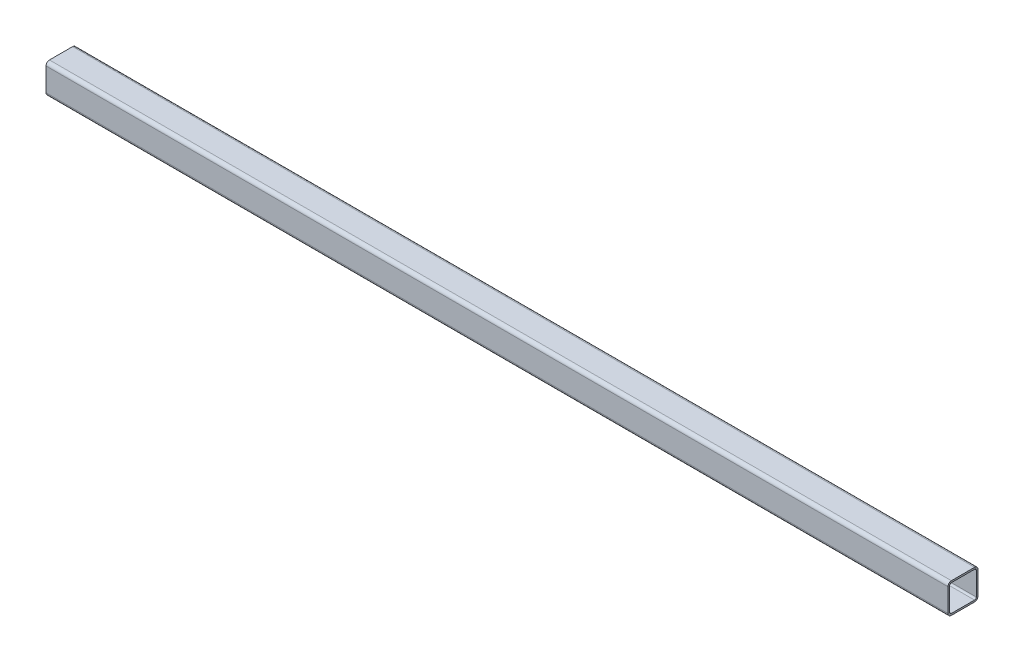
SolidWorks part; units mm, degrees
material "Q235"
ref_plane "Front" through (0, 0, 0) normal (0, 0, 1) x (1, 0, 0)
ref_plane "Top" through (0, 0, 0) normal (0, 1, 0) x (1, 0, 0)
ref_plane "Right" through (0, 0, 0) normal (1, 0, 0) x (0, 0, -1)
sketch "Sketch1" plane through (0, 0, 0) normal (0, 0, 1) x (1, 0, 0)
  line L0 (0, 0) -> (1200, 0)
  dimension "D1" = 1200
other "Square Tube 40 X 40 X 2.3(1)"
ref_plane "Plane1" through (0, 0, 0) normal (1, 0, 0) x (0, 1, 0)
sketch "Sketch11" plane through (0, 0, 0) normal (1, 0, 0) x (0, 1, 0)
  line L0 (-15.4, -17.7) -> (15.4, -17.7)
  line L1 (-17.7, -15.4) -> (-17.7, 15.4)
  line L2 (15.4, 17.7) -> (-15.4, 17.7)
  line L3 (17.7, 15.4) -> (17.7, -15.4)
  line L4 (-15.4, -20) -> (15.4, -20)
  line L5 (-20, -15.4) -> (-20, 15.4)
  line L6 (15.4, 20) -> (-15.4, 20)
  line L7 (20, 15.4) -> (20, -15.4)
  line L8 (-20, 0) -> (-17.7, 0) construction
  line L9 (-17.7, 0) -> (17.7, 0) construction
  line L10 (17.7, 0) -> (20, 0) construction
  line L12 (0, 20) -> (0, 17.7) construction
  line L13 (0, 17.7) -> (0, -17.7) construction
  line L14 (0, -17.7) -> (0, -20) construction
  arc A0 (20, 15.4) -> (15.4, 20) centre (15.4, 15.4) ccw
  arc A1 (15.4, -20) -> (20, -15.4) centre (15.4, -15.4) ccw
  arc A2 (-20, -15.4) -> (-15.4, -20) centre (-15.4, -15.4) ccw
  arc A3 (-15.4, 20) -> (-20, 15.4) centre (-15.4, 15.4) ccw
  arc A4 (-15.4, 17.7) -> (-17.7, 15.4) centre (-15.4, 15.4) ccw
  arc A5 (17.7, 15.4) -> (15.4, 17.7) centre (15.4, 15.4) ccw
  arc A6 (15.4, -17.7) -> (17.7, -15.4) centre (15.4, -15.4) ccw
  arc A7 (-17.7, -15.4) -> (-15.4, -17.7) centre (-15.4, -15.4) ccw
  point P2 (-20, 20)
  point P33 (-20, -20)
  point P34 (20, -20)
  point P36 (20, 20)
  point P37 (0, 0)
  dimension "D1" = 4.6
  dimension "Thickness" = 2.3
  dimension "V_leg" = 40
  dimension "H_leg" = 40
